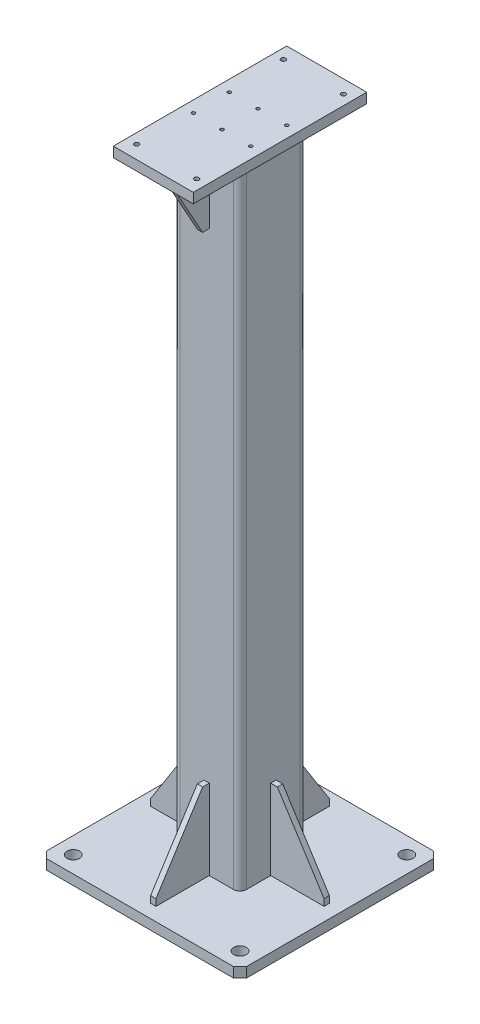
SolidWorks part; units mm, degrees
material "Q235-A"
ref_plane "前视基准面" through (0, 0, 0) normal (0, 0, 1) x (1, 0, 0)
ref_plane "上视基准面" through (0, 0, 0) normal (0, 1, 0) x (1, 0, 0)
ref_plane "右视基准面" through (0, 0, 0) normal (1, 0, 0) x (0, 0, -1)
sketch "草图2" plane through (0, 0, 0) normal (0, 0, 1) x (1, 0, 0)
  line L0 (0, 0) -> (0, 940)
  dimension "D1" = 940
other "方形管 100 X 100 X 5(1)"
ref_plane "基准面1" through (0, 0, 0) normal (0, 1, 0) x (-1, 0, 0)
sketch "Sketch12" plane through (0, 0, 0) normal (0, 1, 0) x (-1, 0, 0)
  line L0 (-40, -45) -> (40, -45)
  line L1 (-45, -40) -> (-45, 40)
  line L2 (40, 45) -> (-40, 45)
  line L3 (45, 40) -> (45, -40)
  line L4 (-40, -50) -> (40, -50)
  line L5 (-50, -40) -> (-50, 40)
  line L6 (40, 50) -> (-40, 50)
  line L7 (50, 40) -> (50, -40)
  arc A0 (50, 40) -> (40, 50) centre (40, 40) ccw
  arc A1 (40, -50) -> (50, -40) centre (40, -40) ccw
  arc A2 (-50, -40) -> (-40, -50) centre (-40, -40) ccw
  arc A3 (-40, 50) -> (-50, 40) centre (-40, 40) ccw
  arc A4 (-40, 45) -> (-45, 40) centre (-40, 40) ccw
  arc A5 (45, 40) -> (40, 45) centre (40, 40) ccw
  arc A6 (40, -45) -> (45, -40) centre (40, -40) ccw
  arc A7 (-45, -40) -> (-40, -45) centre (-40, -40) ccw
  point P0 (-50, 0)
  point P1 (50, 0)
  point P2 (0, 50)
  point P3 (0, -50)
  point P4 (0, 0)
  point P5 (-50, -50)
  point P6 (50, -50)
  point P7 (50, 50)
  point P8 (-50, 50)
  point P33 (0, 0)
  dimension "D1" = 10
  dimension "Thickness" = 5
  dimension "V_leg" = 100
sketch "草图4" plane through (0, 0, 0) normal (0, -1, 0) x (1, 0, 0)
  line L1 (-150, 150) -> (150, 150)
  line L2 (-150, 150) -> (-150, -150)
  line L3 (-150, -150) -> (150, -150)
  line L4 (150, 150) -> (150, -150)
  line L5 (-150, 150) -> (150, -150) construction
  line L6 (-150, -150) -> (150, 150) construction
  point P0 (0, 0)
  dimension "D1" = 300
extrude "凸台-拉伸1" add sketch "草图4" along normal blind 15 separate body
sketch "草图5" plane through (0, 940, 0) normal (0, 1, 0) x (1, 0, 0)
  line L1 (-60, 130) -> (60, 130)
  line L2 (-60, 130) -> (-60, -130)
  line L3 (-60, -130) -> (60, -130)
  line L4 (60, 130) -> (60, -130)
  line L5 (-60, 130) -> (60, -130) construction
  line L6 (-60, -130) -> (60, 130) construction
  point P0 (0, 0)
  dimension "D1" = 260
  dimension "D2" = 120
extrude "凸台-拉伸2" add sketch "草图5" along normal blind 15 separate body
other "角撑板1" parameters "D1"=8, "D2"=5, "D3"=0, "D4"=0, "D10"=5, "D11"=120, "D12"=80, "D13"=10, "D14"=57.529, "D15"=10, "D16"=60, "D17"=40, "D18"=33.69
sketch "草图6" plane through (50, 0, 0) normal (0, 0, -1) x (-1, 0, 0)
  line L0 (0, 0) -> (0, 120)
  line L1 (0, 0) -> (-80, 0)
  line L2 (-10, 120) -> (-80, 10)
  line L3 (0, 120) -> (-10, 120)
  line L4 (-80, 0) -> (-80, 10)
other "角撑板2" parameters "D1"=8, "D2"=8, "D3"=0, "D4"=0, "D10"=5, "D11"=120, "D12"=80, "D13"=10, "D14"=57.529, "D15"=10, "D16"=60, "D17"=40, "D18"=33.69
sketch "草图7" plane through (0, 0, -50) normal (-1, 0, 0) x (0, 0, 1)
  line L0 (0, 0) -> (0, 120)
  line L1 (0, 0) -> (-80, 0)
  line L2 (-10, 120) -> (-80, 10)
  line L3 (0, 120) -> (-10, 120)
  line L4 (-80, 0) -> (-80, 10)
other "角撑板3" parameters "D1"=8, "D2"=8, "D3"=0, "D4"=0, "D10"=5, "D11"=120, "D12"=80, "D13"=10, "D14"=57.529, "D15"=10, "D16"=60, "D17"=40, "D18"=33.69
sketch "草图8" plane through (-50, 0, 0) normal (0, 0, 1) x (1, 0, 0)
  line L0 (0, 0) -> (0, 120)
  line L1 (0, 0) -> (-80, 0)
  line L2 (-10, 120) -> (-80, 10)
  line L3 (0, 120) -> (-10, 120)
  line L4 (-80, 0) -> (-80, 10)
other "角撑板4" parameters "D1"=8, "D2"=8, "D3"=0, "D4"=0, "D10"=5, "D11"=120, "D12"=80, "D13"=10, "D14"=57.529, "D15"=10, "D16"=60, "D17"=40, "D18"=33.69
sketch "草图9" plane through (0, 0, 50) normal (1, 0, 0) x (0, 0, -1)
  line L0 (0, 0) -> (0, 120)
  line L1 (0, 0) -> (-80, 0)
  line L2 (-10, 120) -> (-80, 10)
  line L3 (0, 120) -> (-10, 120)
  line L4 (-80, 0) -> (-80, 10)
other "角撑板5" parameters "D1"=8, "D2"=8, "D3"=0, "D4"=0, "D10"=5, "D11"=100, "D12"=60, "D13"=10, "D14"=60.945, "D15"=10, "D16"=50, "D17"=30, "D18"=30.964
sketch "草图10" plane through (0, 940, -50) normal (1, 0, 0) x (0, 0, -1)
  line L0 (0, 0) -> (0, -100)
  line L1 (0, 0) -> (60, 0)
  line L2 (10, -100) -> (60, -10)
  line L3 (0, -100) -> (10, -100)
  line L4 (60, 0) -> (60, -10)
other "角撑板6" parameters "D1"=8, "D2"=8, "D3"=0, "D4"=0, "D10"=5, "D11"=100, "D12"=60, "D13"=10, "D14"=60.945, "D15"=10, "D16"=50, "D17"=30, "D18"=30.964
sketch "草图11" plane through (0, 940, 50) normal (-1, 0, 0) x (0, 0, 1)
  line L0 (0, 0) -> (0, -100)
  line L1 (0, 0) -> (60, 0)
  line L2 (10, -100) -> (60, -10)
  line L3 (0, -100) -> (10, -100)
  line L4 (60, 0) -> (60, -10)
hole_wizard "Ø19.0 (19) 直径孔1" positions "草图12" profile "草图13" hole size "Ø19.0" standard "GB"
sketch "草图12" plane through (0, 0, 0) normal (0, 1, 0) x (1, 0, 0)
  point P0 (125, -125)
  point P2 (125, 125)
  point P4 (-125, 125)
  point P6 (-125, -125)
sketch "草图13" plane through (125, 0, 125) normal (1, 0, 0) x (0, 0, 1)
  line L0 (0, 0) -> (0, 33.2082)
  line L1 (0, 33.2082) -> (9.5, 27.5)
  line L2 (9.5, 27.5) -> (9.5, 0)
  line L5 (9.5, 0) -> (0, 0)
  line L10 (0, 33.2082) -> (-9.5, 27.5) construction
  line L11 (0, -6.35) -> (0, 107.95) construction
  dimension "孔直径" = 19
  dimension "孔深度" = 27.5
  dimension "导头角度" = 118
hole_wizard "M8 螺纹孔1" positions "草图14" profile "草图15" tap size "M8" standard "GB"
sketch "草图14" plane through (0, 940, 0) normal (0, -1, 0) x (-1, 0, 0)
  point P0 (-45, -110)
  point P2 (45, -110)
  point P4 (45, 110)
  point P6 (-45, 110)
sketch "草图15" plane through (45, 940, 110) normal (1, 0, 0) x (0, 0, -1)
  line L0 (0, 0) -> (0, 21.7929)
  line L1 (0, 21.7929) -> (3.4, 19.75)
  line L2 (3.4, 19.75) -> (3.4, 0)
  line L5 (3.4, 0) -> (0, 0)
  line L10 (0, 21.7929) -> (-3.4, 19.75) construction
  line L11 (0, -6.35) -> (0, 107.95) construction
  dimension "螺纹孔钻头直径" = 6.8
  dimension "螺纹孔钻头深度" = 19.75
  dimension "导头角度" = 118
sketch "草图16" plane through (0, 955, 0) normal (0, 1, 0) x (1, 0, 0)
  line L0 (60, -130) -> (60, 130) construction
  line L1 (-60, -130) -> (60, -130)
  line L2 (-60, -130) -> (-60, -92)
  line L3 (-60, -92) -> (60, -92)
  line L4 (60, -130) -> (60, -92)
  line L6 (-60, 130) -> (60, 130)
  line L7 (-60, 130) -> (-60, 92)
  line L8 (-60, 92) -> (60, 92)
  line L9 (60, 130) -> (60, 92)
  dimension "D1" = 38
chamfer "倒角1" distance 10 angle 45 4 edges at (-150, -7.5, 150) (150, -7.5, 150) (-150, -7.5, -150) (150, -7.5, -150)
sketch "草图17" plane through (0, 955, 0) normal (0, 1, 0) x (1, 0, 0)
  line L0 (-60, 0) -> (60.0307, 0) construction
  line L1 (-60, 130) -> (-60, -130) construction
  line L2 (-78.5017, 30) -> (76.1929, 30) construction
  line L3 (60, 130) -> (-60, 130) construction
  line L4 (0, 0) -> (0, 170.5681) construction
  line L5 (43, 0) -> (43, 170.5681) construction
  line L6 (-43, 0) -> (-43, 170.5681) construction
  point P15 (-43, 30)
  point P16 (0, 30)
  point P17 (43, 30)
  dimension "D1" = 100
  dimension "D2" = 43
  dimension "D3" = 43
hole_wizard "M6 螺纹孔1" positions "3D草图2" profile "草图19" tap size "M6" standard "GB"
sketch3d "3D草图2"
  line L0 (0, 955, -130) -> (0, 955, -772.0555) construction
  line L1 (60, 955, -130) -> (-60, 955, -130) construction
  point P0 (-43, 955, -27)
  point P2 (0, 955, -27)
  dimension "D1" = 103
  dimension "D2" = 43
  dimension "D3" = 103
sketch "草图19" plane through (-43, 955, -27) normal (1, 0, 0) x (0, 0, 1)
  line L0 (0, 0) -> (0, 16.5022)
  line L1 (0, 16.5022) -> (2.5, 15)
  line L2 (2.5, 15) -> (2.5, 0)
  line L5 (2.5, 0) -> (0, 0)
  line L10 (0, 16.5022) -> (-2.5, 15) construction
  line L11 (0, -6.35) -> (0, 107.95) construction
  dimension "螺纹孔钻头直径" = 5
  dimension "螺纹孔钻头深度" = 15
  dimension "导头角度" = 118
cosmetic thread "孔螺蚊线2" parameters "D1"=12, "D2"=6
cosmetic thread "孔螺蚊线3" parameters "D1"=12, "D2"=6
hole_wizard "M6 螺纹孔2" positions "3D草图3" profile "草图20" tap size "M6" standard "GB"
sketch3d "3D草图3"
  line L0 (60, 955, -130) -> (-60, 955, -130) construction
  line L1 (0, 955, -130) -> (0, 955, -103.6941) construction
  point P0 (43, 955, -27)
  dimension "D1" = 103
  dimension "D2" = 43
sketch "草图20" plane through (43, 955, -27) normal (1, 0, 0) x (0, 0, 1)
  line L0 (0, 0) -> (0, 16.5022)
  line L1 (0, 16.5022) -> (2.5, 15)
  line L2 (2.5, 15) -> (2.5, 0)
  line L5 (2.5, 0) -> (0, 0)
  line L10 (0, 16.5022) -> (-2.5, 15) construction
  line L11 (0, -6.35) -> (0, 107.95) construction
  dimension "螺纹孔钻头直径" = 5
  dimension "螺纹孔钻头深度" = 15
  dimension "导头角度" = 118
cosmetic thread "孔螺蚊线4" parameters "D1"=12, "D2"=6
ref_plane "基准面2" through (0, 0, 0) normal (0, 0, 1) x (1, 0, 0)
mirror "镜向1" about plane through (0, 0, 0) normal (0, 0, 1) of "M6 螺纹孔1", "M6 螺纹孔2"
sketch "草图21" plane through (0, 0, 0) normal (0, 1, 0) x (1, 0, 0)
  line L0 (0, 0) -> (-190.0073, -50.9123) construction
  line L1 (-60, -4) -> (-130, -4) construction
  line L2 (0, 0) -> (254.9859, 68.3233) construction
  line L3 (0, 0) -> (-52.3876, 195.5131) construction
  line L4 (0, 0) -> (51.4933, -192.1757) construction
  circle A0 centre (0, 0) radius 137 construction
  point P7 (-132.3318, -35.4582)
  point P8 (132.3318, 35.4582)
  point P11 (35.4582, -132.3318)
  point P12 (-35.4582, 132.3318)
  dimension "D1" = 274
  dimension "D2" = 15
sketch "草图23" [suppressed] plane through (0, 0, 0) normal (0, 1, 0) x (1, 0, 0)
  line L1 (-139.4903, -133) -> (139.4903, -133)
  line L2 (-139.4903, -133) -> (-139.4903, 133)
  line L3 (-139.4903, 133) -> (139.4903, 133)
  line L4 (139.4903, -133) -> (139.4903, 133)
  line L5 (-139.4903, -133) -> (139.4903, 133) construction
  line L6 (-139.4903, 133) -> (139.4903, -133) construction
  point P0 (0, 0)
extrude "切除-拉伸1" [suppressed] cut sketch "草图23" along normal up to surface (940 mm away)
sketch "草图24" [suppressed] plane through (0, 0, 0) normal (0, 1, 0) x (1, 0, 0)
  line L0 (-40, 55) -> (40, 55)
  line L1 (-40, 60) -> (40, 60)
  line L2 (-50, 50) -> (-50, -50)
  line L3 (-40, -60) -> (40, -60)
  line L4 (50, 50) -> (50, -50)
  line L5 (-50, 60) -> (50, -60) construction
  line L6 (-50, -60) -> (50, 60) construction
  line L7 (45, 50) -> (45, -50)
  line L8 (-40, -55) -> (40, -55)
  line L9 (-45, 50) -> (-45, -50)
  arc A0 (50, -50) -> (40, -60) centre (40, -50) cw
  arc A1 (-40, -60) -> (-50, -50) centre (-40, -50) cw
  arc A2 (-50, 50) -> (-40, 60) centre (-40, 50) cw
  arc A3 (50, 50) -> (40, 60) centre (40, 50) ccw
  arc A4 (45, 50) -> (40, 55) centre (40, 50) ccw
  arc A5 (45, -50) -> (40, -55) centre (40, -50) cw
  arc A6 (-40, -55) -> (-45, -50) centre (-40, -50) cw
  arc A7 (-45, 50) -> (-40, 55) centre (-40, 50) cw
  point P0 (0, 0)
  dimension "D3" = 10
  dimension "D4" = 10
  dimension "D1" = 120
  dimension "D2" = 100
  dimension "D5" = 5
extrude "凸台-拉伸4" [suppressed] add sketch "草图24" along normal up to surface (940 mm away) separate body
other "角撑板7" parameters "D1"=8, "D2"=10, "D3"=0, "D4"=0, "D10"=5, "D11"=120, "D12"=80, "D13"=15, "D14"=30, "D15"=82.4722, "D16"=60, "D17"=40, "D18"=33.69
sketch "草图25" plane through (0, 0, 60) normal (1, 0, 0) x (0, 0, -1)
  line L0 (0, 0) -> (0, 120)
  line L1 (0, 0) -> (-80, 0)
  line L2 (0, 120) -> (-80, 0)
other "角撑板8" parameters "D1"=10, "D2"=10, "D3"=0, "D4"=0, "D10"=5, "D11"=120, "D12"=80, "D13"=15, "D14"=30, "D15"=82.4722, "D16"=60, "D17"=40, "D18"=33.69
sketch "草图26" plane through (50, 0, 0) normal (0, 0, -1) x (-1, 0, 0)
  line L0 (0, 0) -> (0, 120)
  line L1 (0, 0) -> (-80, 0)
  line L2 (0, 120) -> (-80, 0)
other "角撑板9" parameters "D1"=10, "D2"=10, "D3"=0, "D4"=0, "D10"=5, "D11"=120, "D12"=80, "D13"=15, "D14"=30, "D15"=82.4722, "D16"=60, "D17"=40, "D18"=33.69
sketch "草图27" plane through (0, 0, -60) normal (-1, 0, 0) x (0, 0, 1)
  line L0 (0, 0) -> (0, 120)
  line L1 (0, 0) -> (-80, 0)
  line L2 (0, 120) -> (-80, 0)
other "角撑板10" parameters "D1"=10, "D2"=10, "D3"=0, "D4"=0, "D10"=5, "D11"=120, "D12"=80, "D13"=15, "D14"=30, "D15"=82.4722, "D16"=60, "D17"=40, "D18"=33.69
sketch "草图28" plane through (-50, 0, 0) normal (0, 0, 1) x (1, 0, 0)
  line L0 (0, 0) -> (0, 120)
  line L1 (0, 0) -> (-80, 0)
  line L2 (0, 120) -> (-80, 0)
other "角撑板11" parameters "D1"=10, "D2"=10, "D3"=0, "D4"=0, "D10"=5, "D11"=80, "D12"=60, "D13"=15, "D14"=30, "D15"=82.4722, "D16"=40, "D17"=30, "D18"=36.87
sketch "草图29" plane through (0, 940, -60) normal (1, 0, 0) x (0, 0, -1)
  line L0 (0, 0) -> (0, -80)
  line L1 (0, 0) -> (60, 0)
  line L2 (0, -80) -> (60, 0)
other "角撑板12" parameters "D1"=10, "D2"=10, "D3"=0, "D4"=0, "D10"=5, "D11"=80, "D12"=60, "D13"=15, "D14"=30, "D15"=82.4722, "D16"=40, "D17"=30, "D18"=36.87
sketch "草图30" plane through (0, 940, 60) normal (-1, 0, 0) x (0, 0, 1)
  line L0 (0, 0) -> (0, -80)
  line L1 (0, 0) -> (60, 0)
  line L2 (0, -80) -> (60, 0)
chamfer "倒角2" [suppressed] distance 5 angle 45
equation "\"D2@草图12\"=\"D1@草图12\""
equation "\"D3@草图12\"=0.5*\"D1@草图12\""
equation "\"D4@草图12\"=0.5*\"D2@草图12\""
equation "\"D3@草图14\"=0.5*\"D2@草图14\""
equation "\"D4@草图14\"=0.5*\"D1@草图14\""
